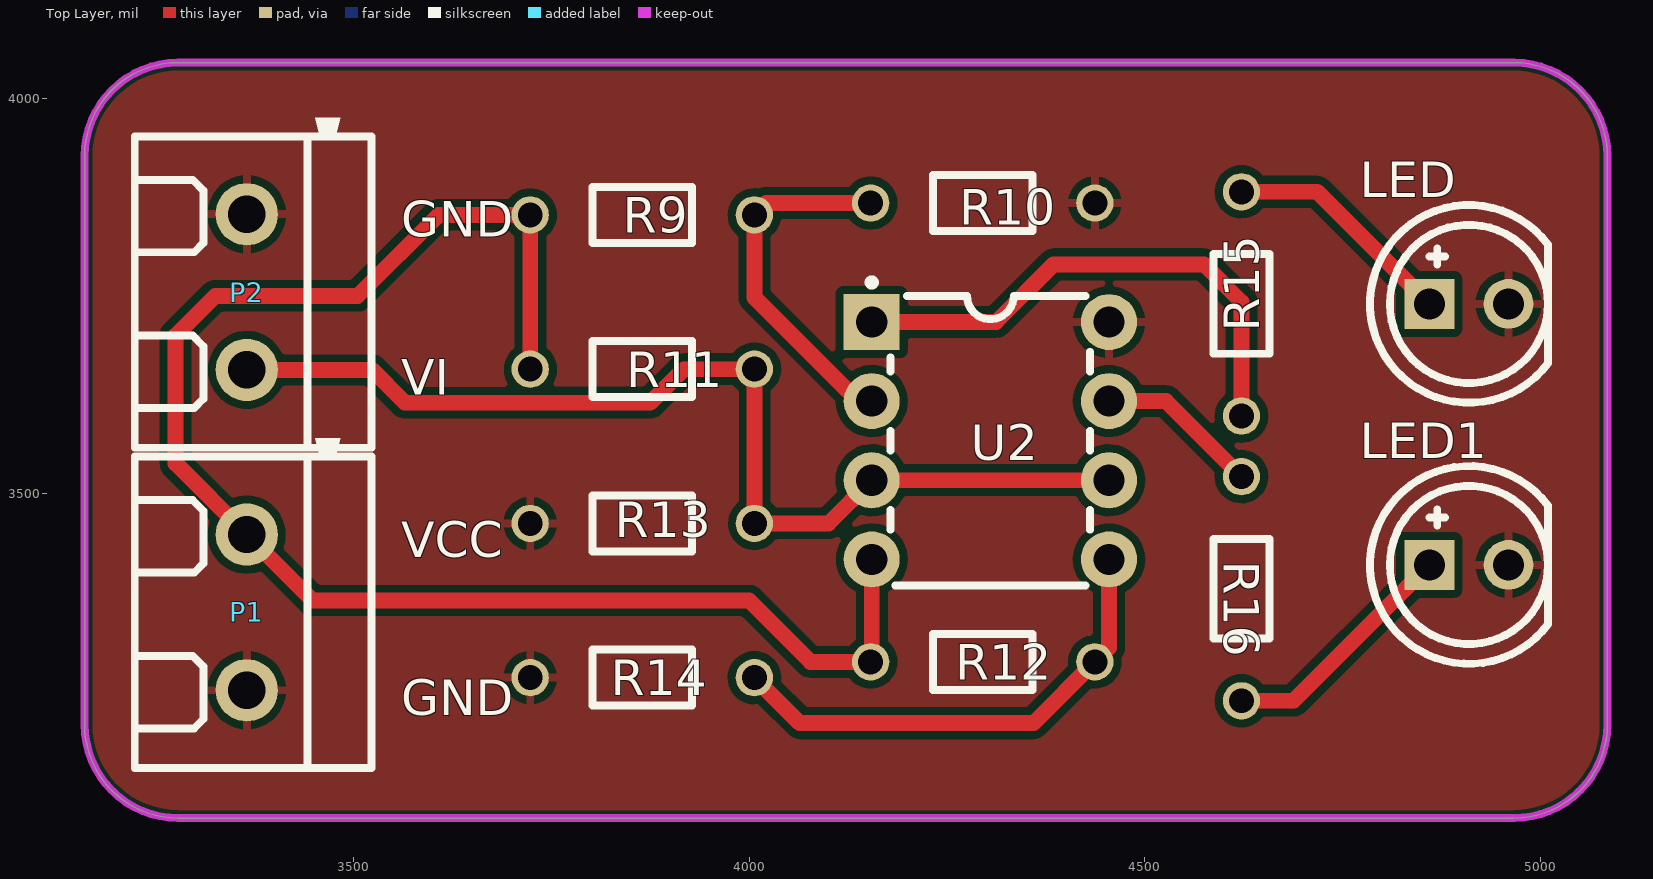
[diagram p0: Top Layer view]
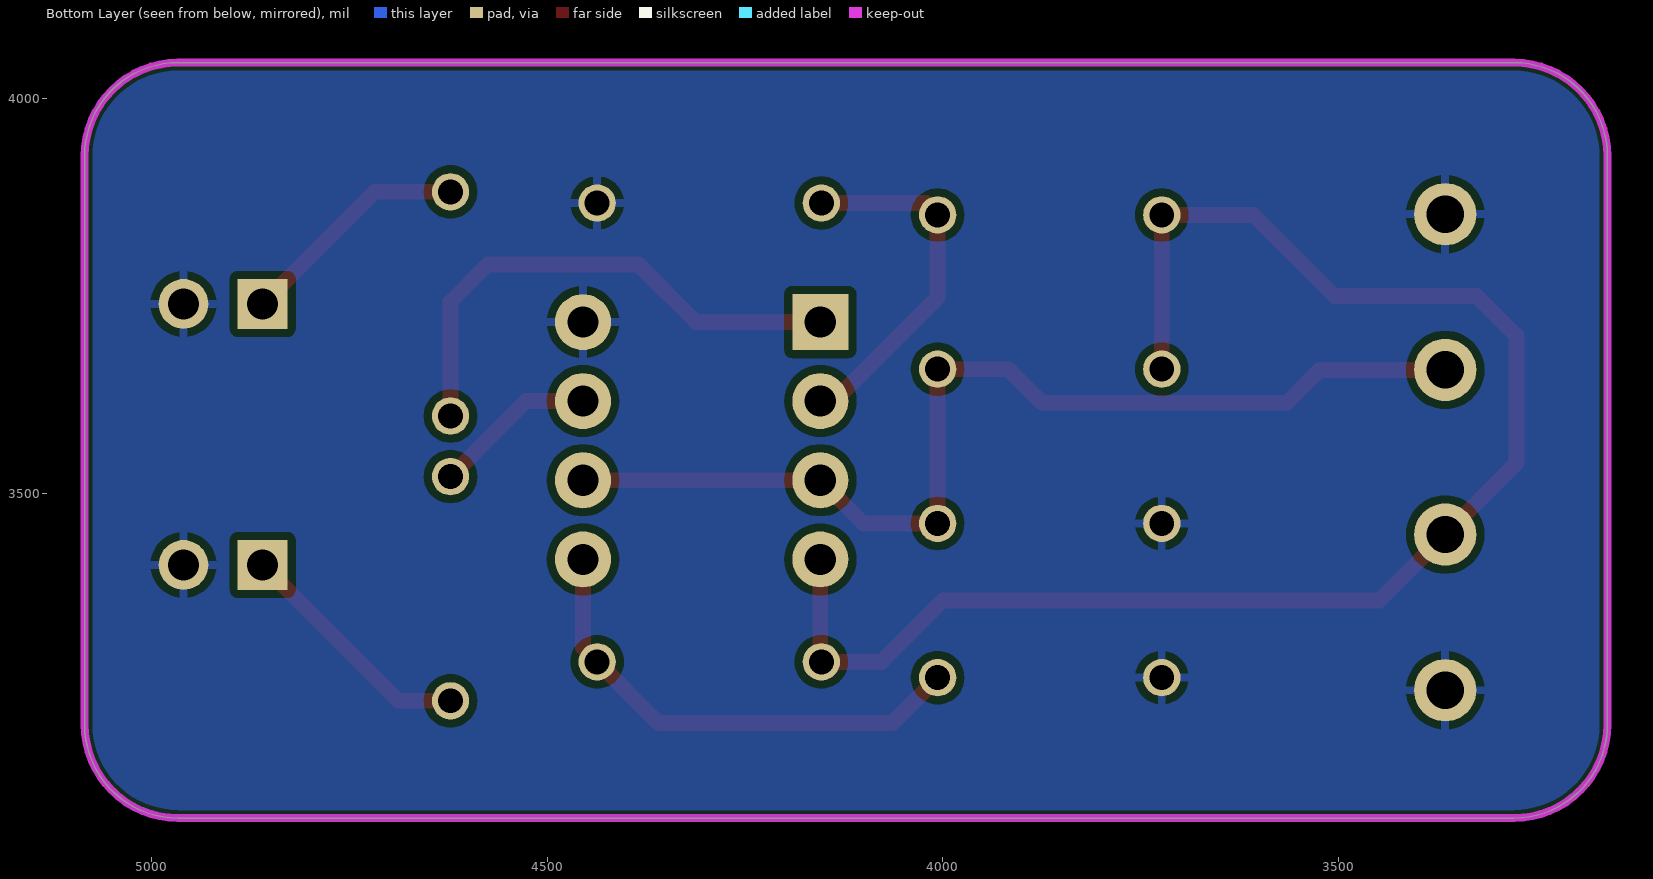
[diagram p1: Bottom Layer view, seen from below]
# Altium PCB MISC50866.pcbdoc
Units mil, origin at the board's own origin, x right, y up, seen from the top; angles counter-clockwise.
Board outline 1925 x 955 mil, 2 copper layers (Top Layer, Bottom Layer), stack 62.206 mil thick; 13 components, 9 nets, 32 pads, 0 vias.

## Layer stack, top to bottom
Top Solder Mask Layer: solder mask 0.394, Dk 3.3
Top Layer: signal copper 1.379
Dielectric1: surface 59.449, FR4, Dk 4.5
Bottom Layer: signal copper 1.378
Bottom Solder Mask Layer: solder mask 0.394, Dk 3.3

## Board outline
3278.11,4045 ccw(c3278.11,3926.89) 3160,3926.89 3160,3208.11 ccw(c3278.11,3208.11) 3278.11,3090 4966.89,3090 ccw(c4966.89,3208.11) 5085,3208.11 5085,3926.89 ccw(c4966.89,3926.89) 4966.89,4045

## Design rules (kind name [scope] priority, off if disabled: settings)
BoardOutlineClearance copperThickness2oz_1 [All] p2 off: genericclearance=7.99 ignorepadtopadclearanceinfootprint=FALSE except(0: Arc-SplitContinuation Track-SplitContinuation SMDPad-SplitContinuation THPad-SplitContinuation Via-SplitContinuation Fill-SplitContinuation Region-SplitContinuation Poly-SplitContinuation Text-SplitContinuation Hole-SplitContinuation; 5.98: Arc-CutoutEdge Track-CutoutEdge SMDPad-CutoutEdge THPad-CutoutEdge Via-CutoutEdge Text-CutoutEdge; 6.9: Hole-OutlineEdge Hole-CutoutEdge; 10: Poly-OutlineEdge Poly-CutoutEdge; 11.81: Arc-OutlineEdge Track-OutlineEdge SMDPad-OutlineEdge THPad-OutlineEdge Via-OutlineEdge Fill-OutlineEdge Region-OutlineEdge Text-OutlineEdge Fill-CutoutEdge Region-CutoutEdge)
BoardOutlineClearance Plane_innerPlane_1 [All] p4 off: genericclearance=4.02 ignorepadtopadclearanceinfootprint=FALSE except(0: Arc-SplitContinuation Track-SplitContinuation SMDPad-SplitContinuation THPad-SplitContinuation Via-SplitContinuation Fill-SplitContinuation Region-SplitContinuation Poly-SplitContinuation Text-SplitContinuation Hole-SplitContinuation; 5.98: Arc-CutoutEdge Track-CutoutEdge SMDPad-CutoutEdge THPad-CutoutEdge Via-CutoutEdge Text-CutoutEdge; 6.9: Hole-OutlineEdge Hole-CutoutEdge; 10: Poly-OutlineEdge Poly-CutoutEdge; 11.81: Arc-OutlineEdge Track-OutlineEdge SMDPad-OutlineEdge THPad-OutlineEdge Via-OutlineEdge Fill-OutlineEdge Region-OutlineEdge Text-OutlineEdge Fill-CutoutEdge Region-CutoutEdge)
BoardOutlineClearance Copper_copperRegion_1 [All] p6 off: genericclearance=4.02 ignorepadtopadclearanceinfootprint=FALSE except(0: Arc-SplitContinuation Track-SplitContinuation SMDPad-SplitContinuation THPad-SplitContinuation Via-SplitContinuation Fill-SplitContinuation Region-SplitContinuation Poly-SplitContinuation Text-SplitContinuation Hole-SplitContinuation; 5.98: Arc-CutoutEdge Track-CutoutEdge SMDPad-CutoutEdge THPad-CutoutEdge Via-CutoutEdge Text-CutoutEdge; 6.9: Hole-OutlineEdge Hole-CutoutEdge; 10: Poly-OutlineEdge Poly-CutoutEdge; 11.81: Arc-OutlineEdge Track-OutlineEdge SMDPad-OutlineEdge THPad-OutlineEdge Via-OutlineEdge Fill-OutlineEdge Region-OutlineEdge Text-OutlineEdge Fill-CutoutEdge Region-CutoutEdge)
BoardOutlineClearance copperThickness1oz_1 [All] p8: genericclearance=4.02 ignorepadtopadclearanceinfootprint=FALSE except(0: Arc-SplitContinuation Track-SplitContinuation SMDPad-SplitContinuation THPad-SplitContinuation Via-SplitContinuation Fill-SplitContinuation Region-SplitContinuation Poly-SplitContinuation Text-SplitContinuation Hole-SplitContinuation; 5.98: Arc-CutoutEdge Track-CutoutEdge SMDPad-CutoutEdge THPad-CutoutEdge Via-CutoutEdge Text-CutoutEdge; 6.9: Hole-OutlineEdge Hole-CutoutEdge; 10: Poly-OutlineEdge Poly-CutoutEdge; 11.81: Arc-OutlineEdge Track-OutlineEdge SMDPad-OutlineEdge THPad-OutlineEdge Via-OutlineEdge Fill-OutlineEdge Region-OutlineEdge Text-OutlineEdge Fill-CutoutEdge Region-CutoutEdge)
Clearance copperThickness2oz [All] p1 off: gap=7.99 ignorepadtopadclearanceinfootprint=FALSE except(5.98: SMDPad-Track SMDPad-SMDPad THPad-Track SMDPad-THPad THPad-THPad Track-Via SMDPad-Via THPad-Via Via-Via Fill-SMDPad Region-SMDPad Fill-THPad Region-THPad Fill-Via Region-Via Fill-Fill Fill-Region Region-Region Arc-Track Arc-SMDPad Arc-THPad Arc-Via Fill-Arc Region-Arc Arc-Arc Text-Track SMDPad-Text Text-THPad Text-Via Fill-Text Region-Text Arc-Text Text-Text; 6.9: Hole-Track Hole-SMDPad Hole-THPad Hole-Via Fill-Hole Region-Hole Hole-Arc Hole-Text; 10: Poly-Track Poly-SMDPad Poly-THPad Poly-Via Poly-Fill Poly-Region Poly-Poly Poly-Arc Poly-Text Poly-Hole; 11.81: Fill-Track Region-Track)
Clearance Plane_innerPlane [All] p3 off: gap=4.02 ignorepadtopadclearanceinfootprint=FALSE except(5.98: SMDPad-Track SMDPad-SMDPad THPad-Track SMDPad-THPad THPad-THPad Track-Via SMDPad-Via THPad-Via Via-Via Fill-SMDPad Region-SMDPad Fill-THPad Region-THPad Fill-Via Region-Via Fill-Fill Fill-Region Region-Region Arc-Track Arc-SMDPad Arc-THPad Arc-Via Fill-Arc Region-Arc Arc-Arc Text-Track SMDPad-Text Text-THPad Text-Via Fill-Text Region-Text Arc-Text Text-Text; 6.9: Hole-Track Hole-SMDPad Hole-THPad Hole-Via Fill-Hole Region-Hole Hole-Arc Hole-Text; 10: Poly-Track Poly-SMDPad Poly-THPad Poly-Via Poly-Fill Poly-Region Poly-Poly Poly-Arc Poly-Text Poly-Hole; 11.81: Fill-Track Region-Track)
Clearance Copper_copperRegion [All] p5 off: gap=4.02 ignorepadtopadclearanceinfootprint=FALSE except(5.98: SMDPad-Track SMDPad-SMDPad THPad-Track SMDPad-THPad THPad-THPad Track-Via SMDPad-Via THPad-Via Via-Via Fill-SMDPad Region-SMDPad Fill-THPad Region-THPad Fill-Via Region-Via Fill-Fill Fill-Region Region-Region Arc-Track Arc-SMDPad Arc-THPad Arc-Via Fill-Arc Region-Arc Arc-Arc Text-Track SMDPad-Text Text-THPad Text-Via Fill-Text Region-Text Arc-Text Text-Text; 6.9: Hole-Track Hole-SMDPad Hole-THPad Hole-Via Fill-Hole Region-Hole Hole-Arc Hole-Text; 10: Poly-Track Poly-SMDPad Poly-THPad Poly-Via Poly-Fill Poly-Region Poly-Poly Poly-Arc Poly-Text Poly-Hole; 11.81: Fill-Track Region-Track)
Clearance copperThickness1oz [All] p7: gap=4.02 ignorepadtopadclearanceinfootprint=FALSE except(5.98: SMDPad-Track SMDPad-SMDPad THPad-Track SMDPad-THPad THPad-THPad Track-Via SMDPad-Via THPad-Via Via-Via Fill-SMDPad Region-SMDPad Fill-THPad Region-THPad Fill-Via Region-Via Fill-Fill Fill-Region Region-Region Arc-Track Arc-SMDPad Arc-THPad Arc-Via Fill-Arc Region-Arc Arc-Arc Text-Track SMDPad-Text Text-THPad Text-Via Fill-Text Region-Text Arc-Text Text-Text; 6.9: Hole-Track Hole-SMDPad Hole-THPad Hole-Via Fill-Hole Region-Hole Hole-Arc Hole-Text; 10: Poly-Track Poly-SMDPad Poly-THPad Poly-Via Poly-Fill Poly-Region Poly-Poly Poly-Arc Poly-Text Poly-Hole; 11.81: Fill-Track Region-Track)
DiffPairsRouting differentialPair [All] p1: maxlimit=6 minlimit=6 mostfreqgap=6 toplayer_minwidth=5 toplayer_prefwidth=10 toplayer_maxwidth=100 toplayer_mingap=6 toplayer_prefgap=6 toplayer_maxgap=6 bottomlayer_minwidth=5 bottomlayer_prefwidth=10 bottomlayer_maxwidth=100 bottomlayer_mingap=6 bottomlayer_prefgap=6 bottomlayer_maxgap=6 maxuncoupledlength=10
HoleToHoleClearance otherClearance [All] p1: gap=11.81 allowstackedmicrovias=TRUE
Length netLength [All] p1: minlimit=0 maxlimit=0
PasteMaskExpansion pasteMaskExpansion [All] p1: expansion=0
PlaneConnect innerPlane [All] p1: planeconnectstyle=Relief reliefexpansion=20 reliefentries=4 reliefconductorwidth=10 reliefairgap=10
PolygonConnect copperRegion [All] p1: connectstyle=Relief reliefconductorwidth=10 reliefentries=4 polygonreliefangle="90 Angle" airgapwidth=10 via.connectstyle=Relief via.reliefconductorwidth=10 via.reliefentries=4 via.polygonreliefangle="90 Angle" via.airgapwidth=10
RoutingVias viaSize [All] p1: holewidth=12.01 width=24.02 viastyle="Through Hole" minholewidth=11.81 minwidth=19.68 maxholewidth=248.03 maxwidth=393.7
SolderMaskExpansion solderMaskExpansion [IsVia] p1: expansion=-1000 istentingtop=TRUE
SolderMaskExpansion solderMaskExpansion [All] p2: expansion=2 istentingtop=FALSE
Width copperThickness2oz_2 [All] p1 off: maxlimit=100 minlimit=8 preferedwidth=10
Width copperThickness1oz_2 [All] p2: maxlimit=100 minlimit=5 preferedwidth=10

## Components (designator, comment, footprint, x,y, rotation, side; value= is the part's Value field where it differs from the comment)
LED "" LED-TH_5mm 4910,3740 r0 top
LED1 "" LED-TH_5mm 4910,3410 r0 top
P1 "KF301-2P接线端子" CONN-TH_XY301V-A-5.0-2P 3365,3350 r90 top
P2 "KF301-2P接线端子" CONN-TH_XY301V-A-5.0-2P 3365,3755 r90 top
R9 "30K" Res_1/8W 3865,3850 r0 top
R10 "68K" Res_1/8W 4295.38,3870 r180 top
R11 "30K" Res_1/8W 3865,3659.95 r180 top
R12 "68K" Res_1/8W 4295.38,3285 r0 top
R13 "51K" Res_1/8W 3865,3460 r0 top
R14 "13K" Res_1/8W 3865,3265 r0 top
R15 "220" Res_1/8W 4624.95,3740 r90 top
R16 "220" Res_1/8W 4620,3380 r270 top
U2 "LM324AD" DIP-8_L9.3-W6.4-P2.54-LS7.6-BL 4305,3567.07 r270 top

## Footprints (in the part's own frame and the unit in brackets; to place one, negate y for a bottom-side part, rotate by r counter-clockwise, add the part's x,y. Pads: shape width x height; smd on the part's side, far side on the other; paste and mask are expansions set on the pad)
CONN-TH_XY301V-A-5.0-2P [mm]
  round 2 hole 1.2: 1(-2.5,0) 2(2.5,0)
  silkscreen extent -5,-4 5.6,3.6
DIP-8_L9.3-W6.4-P2.54-LS7.6-BL [mm]
  rect 1.8x1.8 hole 1: 1(-3.81,-3.81)
  round 1.8 hole 1: 2(-1.27,-3.81) 3(1.27,-3.81) 4(3.81,-3.81) 5(3.81,3.81) 6(1.27,3.81) 7(-1.27,3.81) 8(-3.81,3.81)
  silkscreen extent -5.18,-3.91 4.65,3.2
LED-TH_5mm [mm]
  rect 1.6x1.6 hole 1 paste+0 mask+0.051: 1(-1.27,0)
  round 1.6 hole 1 paste+0 mask+0.051: 2(1.27,0)
  silkscreen extent -3.17,-3.17 2.54,3.17
Res_1/8W [mil]
  round 47.2 hole 31.5 paste+0 mask+2: 1(-141.7,2.48) 2(141.7,2.48)
  silkscreen extent -63,-33 63,38

## Nets (pads, with @x,y where several pads share a name; then routed paths per layer and width w, separated by ;. In a path a pad name is that pad's centre, name@x,y a point inside that pad or via, vN(x,y) a via of type N, cw(c..) or ccw(c..) an arc to the next point about the centre after c; other vN are vias at no path point)
$1N193: R9.2 R10.2 U2.2 | length 460
  Top Layer w20: R10.2 4021.75,3867.52 R9.2 4006.7,3748.3 4137.93,3617.07 U2.2
$1N797: R12.2 R14.2 U2.5 | length 623.3
  Top Layer w20: R14.2 4064.18,3210 4359.6,3210 R12.2 4455,3305.4 U2.5
$1N964: LED.1 R15.2 | length 296.2
  Top Layer w20: R15.2 4718.3,3881.7 LED.1
$1N967: R15.1 U2.1 | length 661.6
  Top Layer w20: U2.1 4312.07,3717.07 4385,3790 4575,3790 4622.48,3742.52 R15.1
$1N1018: LED1.1 R16.2 | length 308.6
  Top Layer w20: R16.2 4688.3,3238.3 LED1.1
$1N1021: R16.1 U2.7 | length 207
  Top Layer w20: U2.7 4527.11,3617.07 R16.1
GND: LED1.2 LED.2 P1.1 P2.2 R10.1 R13.1 R14.1 U2.8
VCC: P1.2 R9.1 R11.2 R12.1 U2.4 | length 1980.8
  Top Layer w20: R11.2 R9.1 3607.48,3852.48 3505,3750 3325,3750 3275,3700 3275,3538.43 P1.2 3448.43,3365 4000,3365 4077.52,3287.48 R12.1 4155,3288.8 U2.4
VI: P2.1 R11.1 R13.2 U2.3 U2.6 | length 1342.4
  Top Layer w20: P2.1 3523.43,3656.57 3565,3615 3875,3615 3917.48,3657.48 R11.1 R13.2 4100.41,3462.48 U2.3 U2.6

## Polygon pours and split planes (outlines as drawn)
GND on Top Layer (solid, remove dead copper, pour order 0): 3010,4205 3010,3005 5310,3005 5310,4205
GND on Bottom Layer (solid, remove dead copper, pour order 2): 3000,4170 3000,3000 5455,3000 5455,4170

## Keep-outs
Board Outline Layer:
  the board outline again, w10

## Silkscreen, mask and mechanical layers (free items; w line width, h text height)
Top Silkscreen Layer:
  text "GND" at 3560,3825 h45
  text "VI" at 3560,3625 h45
  text "VCC" at 3560,3420 h45
  text "GND" at 3560,3220 h45